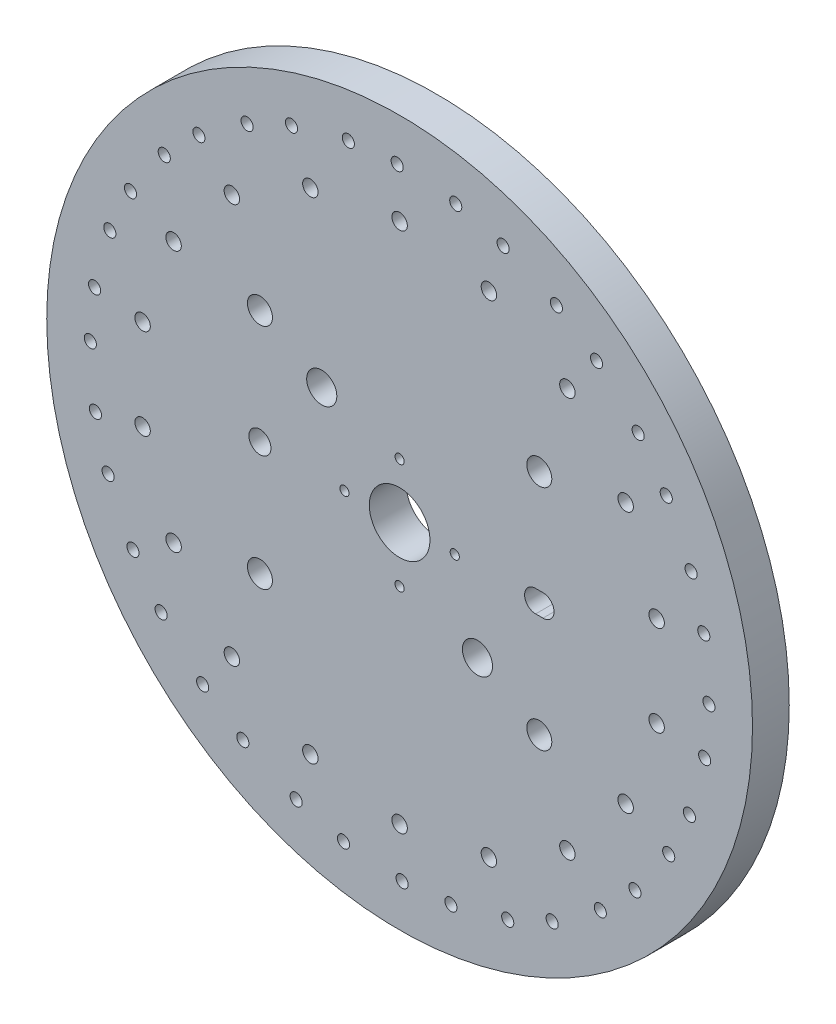
from build123d import *

# Parameters (mm, degrees)
SKETCH1_R           = 102.5
BOSS_EXTRUDE1_DEPTH = 10
SKETCH2_R           = 8.25
CUT_EXTRUDE1_DEPTH  = 146.301410867
SKETCH4_R           = 1
CUT_EXTRUDE3_DEPTH  = 20
CIRPATTERN2_COUNT   = 18
SKETCH5_R           = 2.1
CUT_EXTRUDE4_DEPTH  = 146.301410867
CIRPATTERN3_COUNT   = 18
SKETCH7_R           = 102.5
SKETCH7_R_2         = 96
CUT_EXTRUDE5_DEPTH  = 34
M4_TAPPED_HOLE1_D   = 3.3
M8_TAPPED_HOLE2_D   = 6.8
M3_TAPPED_HOLE1_D   = 2.5
SKETCH44_R          = 4.1
CUT_EXTRUDE19_DEPTH = 10
SKETCH45_R          = 3
CUT_EXTRUDE20_DEPTH = 10
CUT_EXTRUDE21_DEPTH = 137.132288602


with BuildPart() as part:
    # Sketch1 → Boss-Extrude1 (new body)
    with BuildSketch(Plane.XY):
        Circle(SKETCH1_R)
    extrude(amount=BOSS_EXTRUDE1_DEPTH)

    # Sketch2 → Cut-Extrude1 (cut, through all)
    with BuildSketch(Plane(origin=(0, 0, 0), x_dir=(-1, 0, 0), z_dir=(0, 0, -1))):
        Circle(SKETCH2_R)
    extrude(amount=-CUT_EXTRUDE1_DEPTH, mode=Mode.SUBTRACT)

    # Sketch4 → Cut-Extrude3 (cut)
    with BuildSketch(Plane(origin=(0, 0, 0), x_dir=(-1, 0, 0), z_dir=(0, 0, -1))):
        with Locations((-29.407083899, -78.839104774)):
            Circle(SKETCH4_R)
        with Locations(Location((-13.952270679, -82.980209495, 0), (0, 0, 180))):
            Circle(SKETCH4_R)
    cut_extrude3 = extrude(amount=-CUT_EXTRUDE3_DEPTH, mode=Mode.SUBTRACT)

    # CirPattern2: Cut-Extrude3 ×18 about axis
    cirpattern2_axis = Axis((0, 0, 0), (0, 0, 1))
    for i in range(1, CIRPATTERN2_COUNT):
        add(cut_extrude3.rotate(cirpattern2_axis, i * 360 / CIRPATTERN2_COUNT), mode=Mode.SUBTRACT)

    # Sketch5 → Cut-Extrude4 (cut, through all)
    with BuildSketch(Plane(origin=(0, 0, 0), x_dir=(-1, 0, 0), z_dir=(0, 0, -1))):
        with Locations((0, -71)):
            Circle(SKETCH5_R)
    cut_extrude4 = extrude(amount=-CUT_EXTRUDE4_DEPTH, mode=Mode.SUBTRACT)

    # CirPattern3: Cut-Extrude4 ×18 about axis
    cirpattern3_axis = Axis((0, 0, 0), (0, 0, 1))
    for i in range(1, CIRPATTERN3_COUNT):
        add(cut_extrude4.rotate(cirpattern3_axis, i * 360 / CIRPATTERN3_COUNT), mode=Mode.SUBTRACT)

    # Sketch7 → Cut-Extrude5 (cut)
    with BuildSketch(Plane(origin=(0, 0, 0), x_dir=(-1, 0, 0), z_dir=(0, 0, -1))):
        Circle(SKETCH7_R)
        Circle(SKETCH7_R_2, mode=Mode.SUBTRACT)
    extrude(amount=-CUT_EXTRUDE5_DEPTH, mode=Mode.SUBTRACT)

    # M4 Tapped Hole1 (through all)
    with Locations(Plane(origin=(-15.270057345, -82.747848151, 10), x_dir=(1, 0, 0), z_dir=(0, 0, 1))):
        with Locations((0, 0), (-12.879609153, 3.451080871), (-27.380533745, 10.212973059), (-38.303068251, 17.861014056), (-49.61677675, 29.174722555), (-57.264817747, 40.097257061), (-64.026709935, 54.598181653), (-67.477790806, 67.477790806), (-68.87228269, 83.416905976), (-67.71015215, 96.70011883), (-63.569047429, 112.15493205), (-57.933875572, 124.239597096), (-48.75665259, 137.346029805), (-39.328124309, 146.774558086), (-26.2216916, 155.951781068), (-14.137026554, 161.586952925), (1.317786666, 165.728057646), (14.60099952, 166.890188186), (30.54011469, 165.495696302), (43.419723843, 162.044615431), (57.920648435, 155.282723243), (68.843182941, 147.634682246), (80.15689144, 136.320973747), (87.804932437, 125.398439241), (94.566824625, 110.897514649), (98.017905496, 98.017905496), (99.41239738, 82.078790326), (98.25026684, 68.795577472), (94.109162119, 53.340764252), (88.473990262, 41.256099206), (79.29676728, 28.149666497), (69.868238999, 18.721138216), (56.76180629, 9.543915234), (44.677141244, 3.908743377), (29.222328024, -0.232361344), (15.93911517, -1.394491884)):
            Hole(M4_TAPPED_HOLE1_D / 2)

    # M8 Tapped Hole2 (through all)
    with Locations(Plane.XY.offset(10)):
        with Locations((-38, 31), (-38, -31), (38, 31), (38, -31)):
            Hole(M8_TAPPED_HOLE2_D / 2)

    # M3 Tapped Hole1 (through all)
    with Locations(Plane(origin=(0, 15, 10), x_dir=(1, 0, 0), z_dir=(0, 0, 1))):
        with Locations((0, 0), (15, -15), (0, -30), (-15, -15)):
            Hole(M3_TAPPED_HOLE1_D / 2)

    # Sketch44 → Cut-Extrude19 (cut)
    with BuildSketch(Plane.XY.offset(10)):
        with Locations((21.183540931, -21.242824521)):
            Circle(SKETCH44_R)
        with Locations((-21.183540931, 21.242824521)):
            Circle(SKETCH44_R)
    extrude(amount=-CUT_EXTRUDE19_DEPTH, mode=Mode.SUBTRACT)

    # Sketch45 → Cut-Extrude20 (cut)
    with BuildSketch(Plane.XY.offset(10)):
        with Locations((-38, 0)):
            Circle(SKETCH45_R)
        with Locations((38, 0)):
            Circle(SKETCH45_R)
    extrude(amount=-CUT_EXTRUDE20_DEPTH, mode=Mode.SUBTRACT)

    # Sketch47 → Cut-Extrude21 (cut, through all)
    with BuildSketch(Plane.XY.offset(10)):
        with BuildLine():
            Line((37, 3), (39, 3))
            ThreePointArc((39, 3), (42, 0), (39, -3))
            Line((39, -3), (37, -3))
            ThreePointArc((37, -3), (34, 0), (37, 3))
        make_face()
    extrude(amount=-CUT_EXTRUDE21_DEPTH, mode=Mode.SUBTRACT)


solid = part.part
